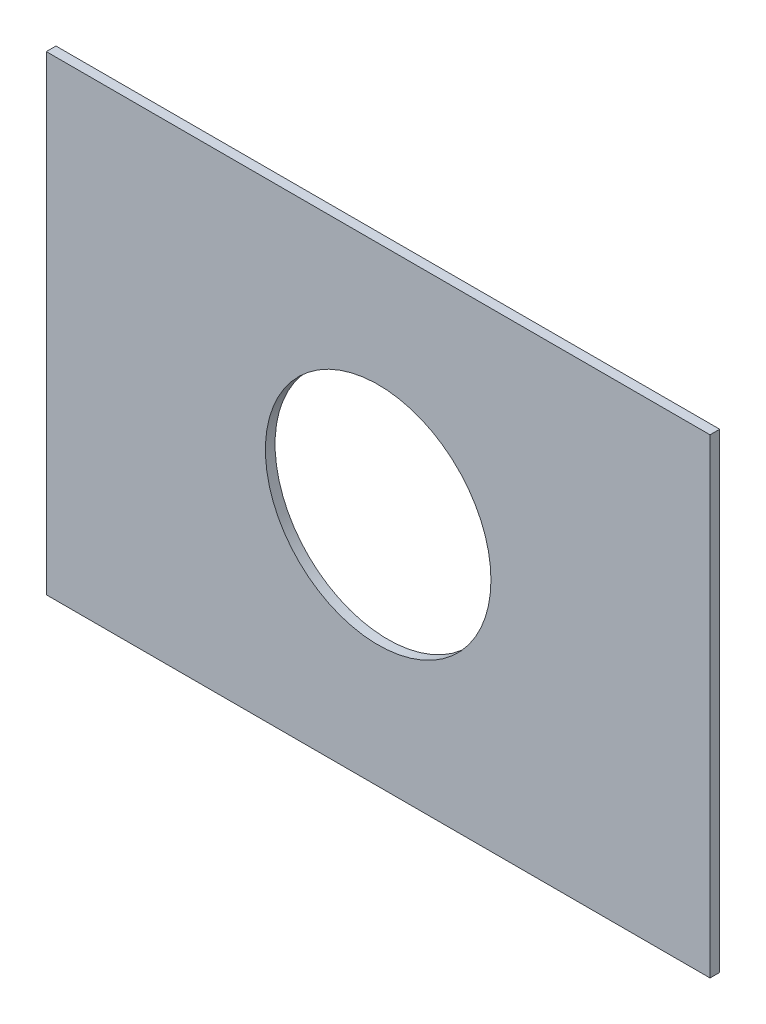
from build123d import *

# Parameters (mm, degrees)
SKETCH_1_W          = 206
SKETCH_1_H          = 146
EXTRUDE_1_DEPTH     = 1.5
SKETCH_2_R          = 35
CUT_EXTRUDE_1_DEPTH = 11.5


with BuildPart() as part:
    # 草图1 → 凸台-拉伸1 (new, symmetric)
    with BuildSketch(Plane.XY):
        Rectangle(SKETCH_1_W, SKETCH_1_H)
    extrude(amount=EXTRUDE_1_DEPTH, both=True)

    # 草图2 → 切除-拉伸1 (cut, symmetric)
    with BuildSketch(Plane.XY):
        Circle(SKETCH_2_R)
    extrude(amount=CUT_EXTRUDE_1_DEPTH, both=True, mode=Mode.SUBTRACT)


solid = part.part
